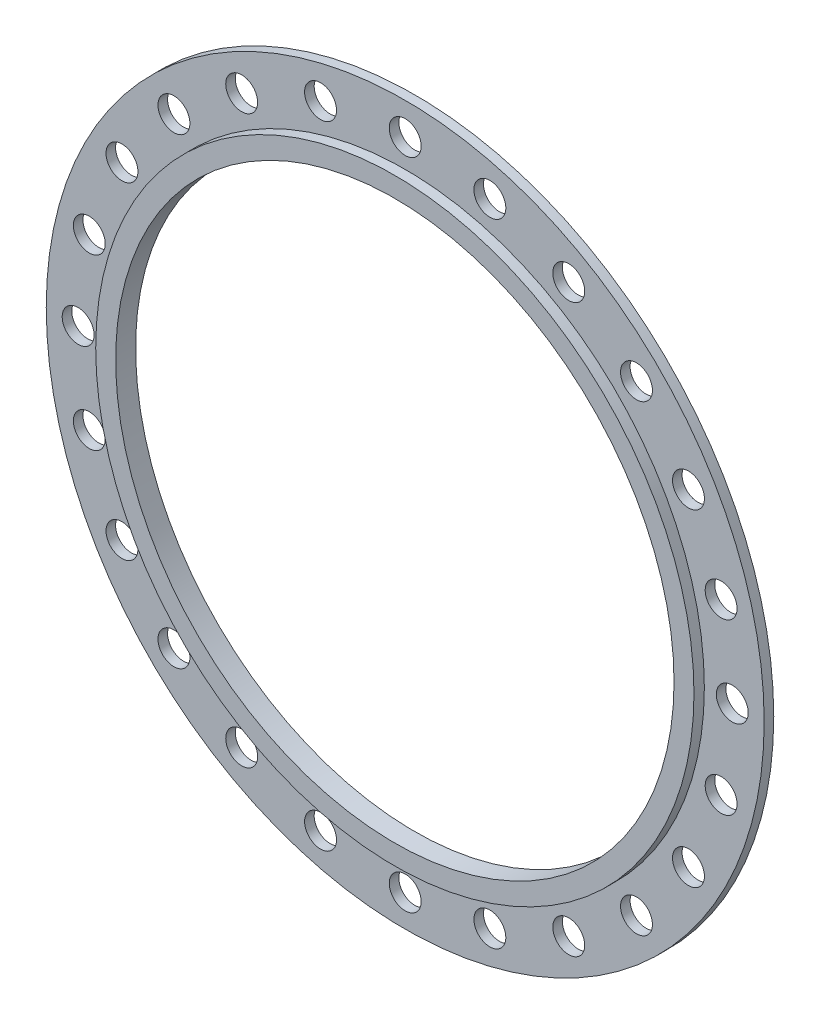
from build123d import *

# Parameters (mm, degrees)
SKETCH_1_R          = 450
EXTRUDE_1_DEPTH     = 12
SKETCH_2_R          = 375
EXTRUDE_2_DEPTH     = 13
SKETCH_3_R          = 20
CUT_EXTRUDE_2_DEPTH = 314
SKETCH_4_R          = 350
CUT_EXTRUDE_3_DEPTH = 314


with BuildPart() as part:
    # 草图1 → 凸台-拉伸1 (new body)
    with BuildSketch(Plane.XY):
        Circle(SKETCH_1_R)
    extrude(amount=EXTRUDE_1_DEPTH)

    # 草图2 → 凸台-拉伸2 (add)
    with BuildSketch(Plane.XY.offset(12)):
        with Locations(Location((0, 0, 0), (0, 0, 180))):
            Circle(SKETCH_2_R)
    extrude(amount=EXTRUDE_2_DEPTH)

    # 草图3 → 切除-拉伸2 (cut)
    with BuildSketch(Plane(origin=(0, 0, 0), x_dir=(-1, 0, 0), z_dir=(0, 0, -1))):
        with Locations((0, 410)):
            Circle(SKETCH_3_R)
        with Locations((106.115808492, 396.029588779)):
            Circle(SKETCH_3_R)
        with Locations((205, 355.070415552)):
            Circle(SKETCH_3_R)
        with Locations((289.913780286, 289.913780286)):
            Circle(SKETCH_3_R)
        with Locations((355.070415552, 205)):
            Circle(SKETCH_3_R)
        with Locations((396.029588779, 106.115808492)):
            Circle(SKETCH_3_R)
        with Locations((410, 0)):
            Circle(SKETCH_3_R)
        with Locations((396.029588779, -106.115808492)):
            Circle(SKETCH_3_R)
        with Locations((355.070415552, -205)):
            Circle(SKETCH_3_R)
        with Locations((289.913780286, -289.913780286)):
            Circle(SKETCH_3_R)
        with Locations((205, -355.070415552)):
            Circle(SKETCH_3_R)
        with Locations((106.115808492, -396.029588779)):
            Circle(SKETCH_3_R)
        with Locations((0, -410)):
            Circle(SKETCH_3_R)
        with Locations((-106.115808492, -396.029588779)):
            Circle(SKETCH_3_R)
        with Locations((-205, -355.070415552)):
            Circle(SKETCH_3_R)
        with Locations((-289.913780286, -289.913780286)):
            Circle(SKETCH_3_R)
        with Locations((-355.070415552, -205)):
            Circle(SKETCH_3_R)
        with Locations((-396.029588779, -106.115808492)):
            Circle(SKETCH_3_R)
        with Locations((-410, 0)):
            Circle(SKETCH_3_R)
        with Locations((-396.029588779, 106.115808492)):
            Circle(SKETCH_3_R)
        with Locations((-355.070415552, 205)):
            Circle(SKETCH_3_R)
        with Locations((-289.913780286, 289.913780286)):
            Circle(SKETCH_3_R)
        with Locations((-205, 355.070415552)):
            Circle(SKETCH_3_R)
        with Locations((-106.115808492, 396.029588779)):
            Circle(SKETCH_3_R)
    extrude(amount=-CUT_EXTRUDE_2_DEPTH, mode=Mode.SUBTRACT)

    # 草图4 → 切除-拉伸3 (cut)
    with BuildSketch(Plane.XY.offset(25)):
        Circle(SKETCH_4_R)
    extrude(amount=-CUT_EXTRUDE_3_DEPTH, mode=Mode.SUBTRACT)


solid = part.part
